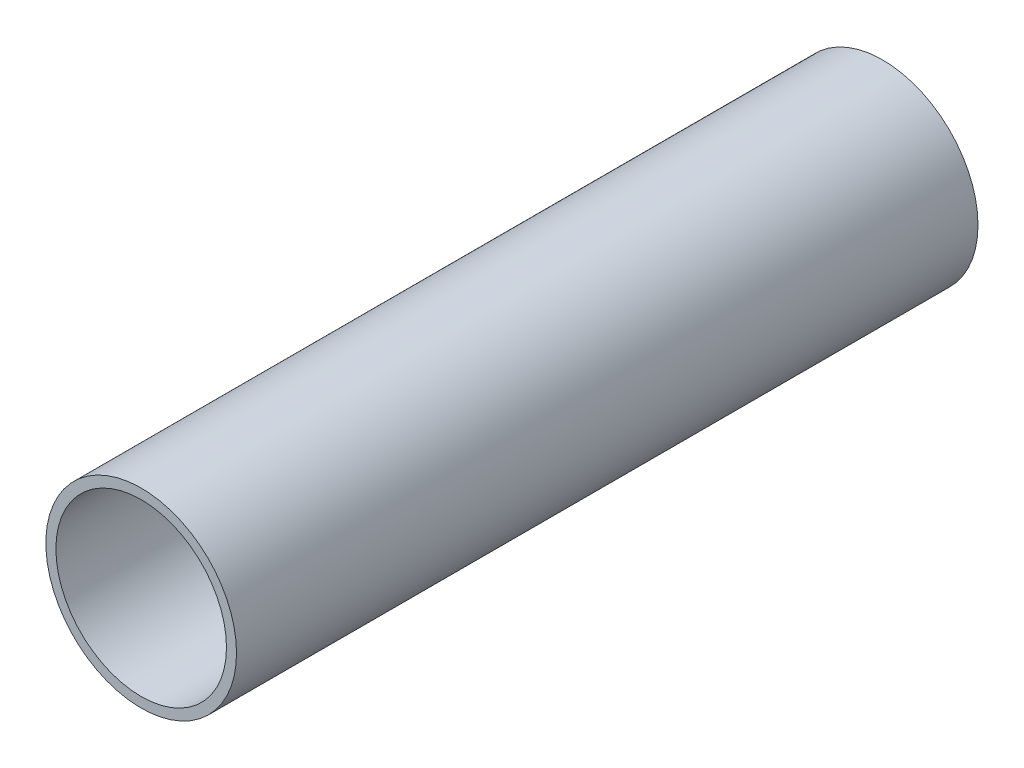
SolidWorks part; units mm, degrees
ref_plane "Front Plane" through (0, 0, 0) normal (0, 0, 1) x (1, 0, 0)
ref_plane "Top Plane" through (0, 0, 0) normal (0, 1, 0) x (1, 0, 0)
ref_plane "Right Plane" through (0, 0, 0) normal (1, 0, 0) x (0, 0, -1)
sketch "Sketch1" plane through (0, 0, 0) normal (0, 0, 1) x (1, 0, 0)
  circle A0 centre (0, 0) radius 57.15
  circle A1 centre (0, 0) radius 51.1302
extrude "Boss-Extrude1" add sketch "Sketch1" along normal up to vertex (222.25 mm away) and the other way up to vertex (222.25 mm away)
